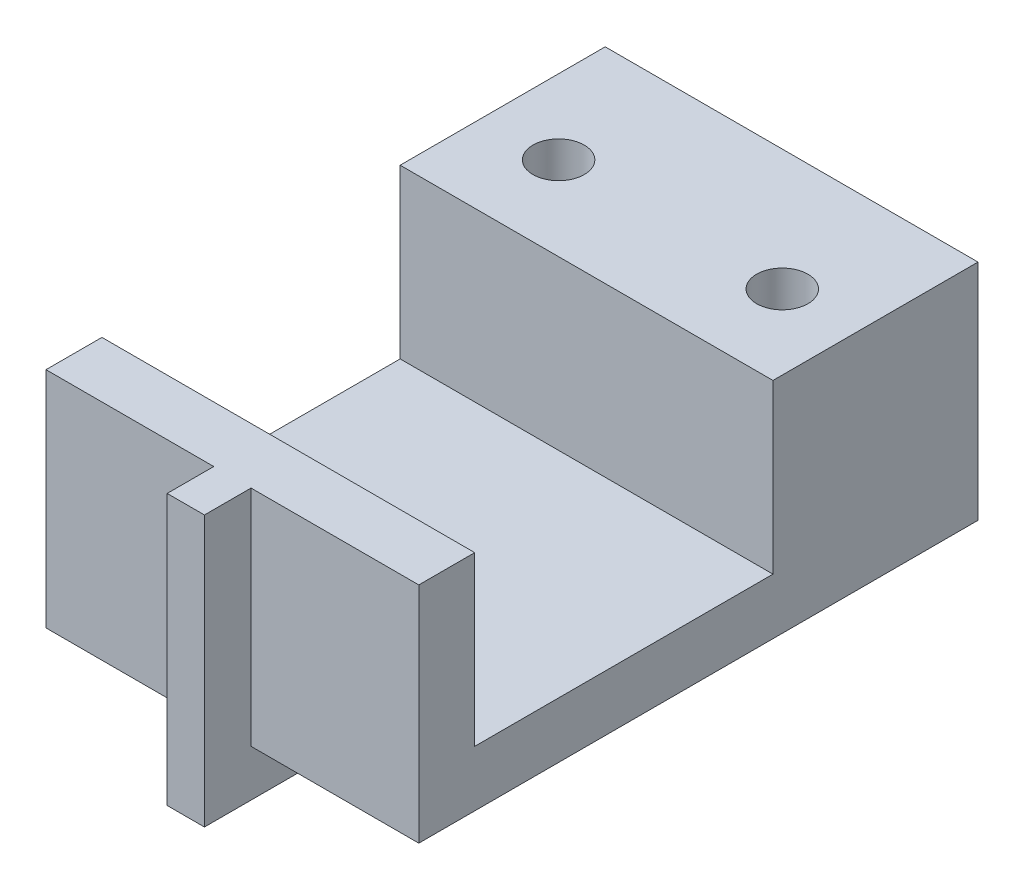
SolidWorks part; units mm, degrees
ref_plane "Front Plane" through (0, 0, 0) normal (0, 0, 1) x (1, 0, 0)
ref_plane "Top Plane" through (0, 0, 0) normal (0, 1, 0) x (1, 0, 0)
ref_plane "Right Plane" through (0, 0, 0) normal (1, 0, 0) x (0, 0, -1)
other "Configuration Table"
sketch "Sketch1" plane through (0, 0, 0) normal (0, 1, 0) x (1, 0, 0)
  line L1 (-20, -30) -> (20, -30)
  line L2 (-20, -30) -> (-20, 30)
  line L3 (-20, 30) -> (20, 30)
  line L4 (20, -30) -> (20, 30)
  line L5 (-20, -30) -> (20, 30) construction
  line L6 (-20, 30) -> (20, -30) construction
  point P0 (0, 0)
  dimension "D1" = 40
  dimension "D2" = 60
extrude "Boss-Extrude1" add sketch "Sketch1" along normal blind 24
sketch "Sketch4" plane through (-20, 0, 0) normal (-1, 0, 0) x (0, 0, 1)
  line L1 (30, 24) -> (-8, 24)
  line L2 (30, 24) -> (30, 6)
  line L3 (30, 6) -> (-8, 6)
  line L4 (-8, 24) -> (-8, 6)
  dimension "D1" = 18
  dimension "D2" = 38
extrude "Cut-Extrude2" cut sketch "Sketch4" against normal blind 83
sketch "Sketch5" plane through (0, 0, 0) normal (0, -1, 0) x (1, 0, 0)
  line L0 (-20, 30) -> (20, 30) construction
  line L1 (-2, -30) -> (2, -30)
  line L2 (-2, -30) -> (-2, 30)
  line L3 (-2, 30) -> (2, 30)
  line L4 (2, -30) -> (2, 30)
  line L5 (-2, -30) -> (2, 30) construction
  line L6 (-2, 30) -> (2, -30) construction
  point P0 (0, 0)
  dimension "D1" = 4
extrude "Boss-Extrude2" add sketch "Sketch5" along normal blind 5
sketch "Sketch6" plane through (0, 0, 30) normal (0, 0, 1) x (1, 0, 0)
  line L0 (20, 6) -> (-20, 6) construction
  line L1 (-2, -5) -> (2, -5)
  line L2 (-2, -5) -> (-2, 6)
  line L3 (-2, 6) -> (2, 6)
  line L4 (2, -5) -> (2, 6)
extrude "Boss-Extrude3" add sketch "Sketch6" along normal blind 5
sketch "Sketch7" plane through (0, 6, 0) normal (0, 1, 0) x (1, 0, 0)
  line L0 (20, 8) -> (20, -30) construction
  line L1 (-20, -30) -> (20, -30)
  line L2 (-20, -30) -> (-20, -24)
  line L3 (-20, -24) -> (20, -24)
  line L4 (20, -30) -> (20, -24)
  dimension "D1" = 6
extrude "Boss-Extrude4" add sketch "Sketch7" along normal up to surface (18 mm away) up to face at (0, 24, -19)
hole_wizard "CBORE for M5 Hexagon socket head cap screws1" positions "Sketch8" profile "Sketch10" counterbore size "M5" standard "GB" end condition through all
sketch "Sketch8" plane through (0, 0, 0) normal (0, -1, 0) x (-1, 0, 0)
  line L0 (-20, 30) -> (-2, 30) construction
  line L1 (2, 30) -> (20, 30) construction
  point P0 (-12, 17)
  point P2 (12, 17)
  dimension "D1" = 13
  dimension "D2" = 13
  dimension "D3" = 24
  dimension "D4" = 12
sketch "Sketch10" plane through (12, 0, -17) normal (1, 0, 0) x (0, 0, -1)
  line L0 (0, 0) -> (0, 24)
  line L1 (0, 24) -> (2.75, 24)
  line L3 (2.75, 24) -> (2.75, 5.7)
  line L4 (5, 5.7) -> (2.75, 5.7)
  line L5 (5, 5.7) -> (5, 0.025)
  line L6 (5, 0.025) -> (5.025, 0)
  line L7 (5.025, 0) -> (0, 0)
  line L8 (-5, 0.025) -> (-5.025, 0) construction
  line L11 (0, -6.35) -> (0, 107.95) construction
  dimension "通孔孔直径" = 5.5
  dimension "通孔孔深度" = 24
  dimension "柱形沉头孔直径" = 10
  dimension "柱形沉头孔深度" = 5.7
  dimension "近端锥形沉头孔直径" = 10.05
  dimension "近端锥形沉头孔角度" = 90
sketch "Sketch11" plane through (0, 6, 0) normal (0, 1, 0) x (1, 0, 0)
  line L4 (2, -30) -> (-2, -30)
  line L5 (-2, -30) -> (-2, -35)
  line L6 (-2, -35) -> (2, -35)
  line L7 (2, -35) -> (2, -30)
  line L8 (2, -30) -> (-2, -30)
  line L9 (-2, -30) -> (-2, -35)
  line L10 (-2, -35) -> (2, -35)
  line L11 (2, -35) -> (2, -30)
  dimension "D1" = 0
extrude "Boss-Extrude5" add sketch "Sketch11" along normal up to surface (18 mm away) up to face at (0, 24, 27)
